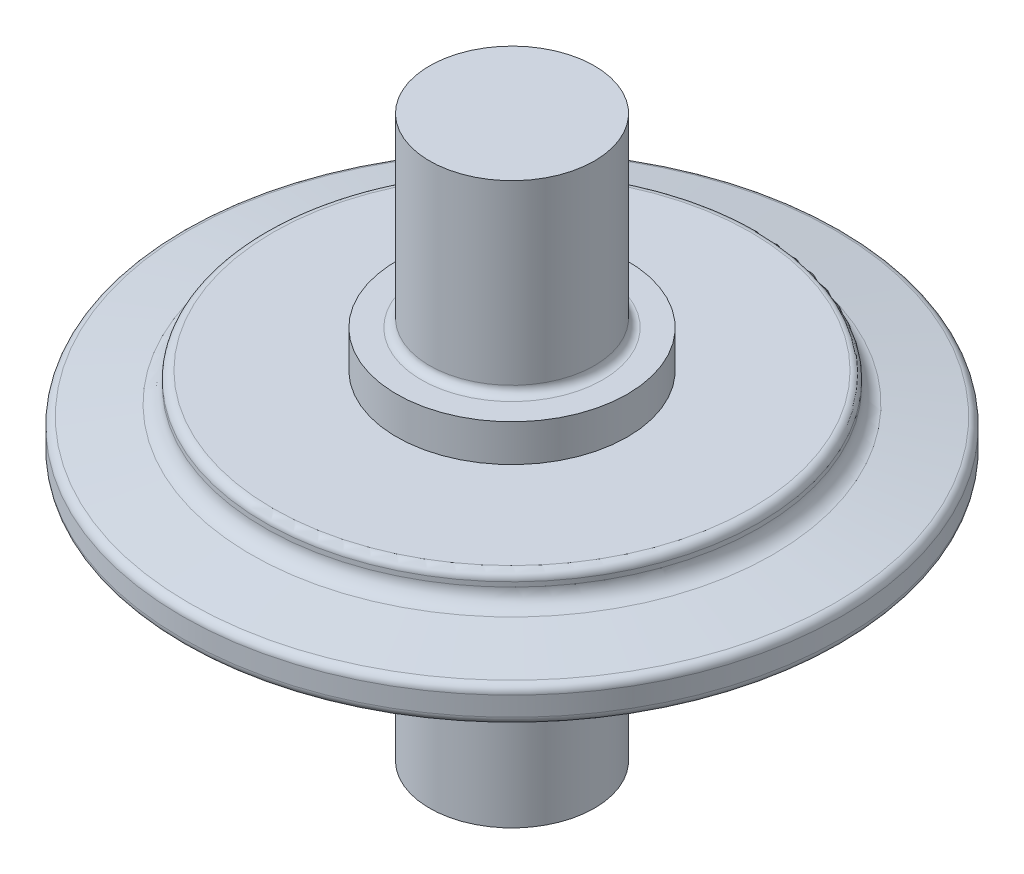
SolidWorks part; units mm, degrees
ref_plane "Front Plane" through (0, 0, 0) normal (0, 0, 1) x (1, 0, 0)
ref_plane "Top Plane" through (0, 0, 0) normal (0, 1, 0) x (1, 0, 0)
ref_plane "Right Plane" through (0, 0, 0) normal (1, 0, 0) x (0, 0, -1)
sketch "Sketch1" plane through (0, 0, 0) normal (0, 0, 1) x (1, 0, 0)
  line L0 (249.7318, 31.6679) -> (249.7318, 29.346)
  line L1 (258.0791, 33.9788) -> (250.5581, 32.6527)
  line L2 (250.5581, 28.3612) -> (258.0791, 27.0351)
  line L3 (259.7318, 25.0655) -> (259.7318, 24.507)
  line L4 (259.7318, 36.507) -> (259.7318, 35.9484)
  line L5 (275.7318, 23.507) -> (275.7318, 19.007)
  line L6 (275.7318, 42.007) -> (275.7318, 37.507)
  line L7 (279.7318, 18.007) -> (279.7318, -3.493)
  line L8 (279.7318, 64.507) -> (279.7318, 43.007)
  line L9 (289.7318, 64.507) -> (279.7318, 64.507)
  line L10 (289.7318, -3.493) -> (279.7318, -3.493)
  line L11 (289.7318, -3.493) -> (289.7318, 64.507)
  line L12 (260.7318, 23.507) -> (275.7318, 23.507)
  line L13 (260.7318, 37.507) -> (275.7318, 37.507)
  line L14 (275.7318, 19.007) -> (278.7318, 19.007)
  line L15 (275.7318, 42.007) -> (278.7318, 42.007)
  arc A1 (249.7318, 29.346) -> (250.5581, 28.3612) centre (250.7318, 29.346) ccw
  arc A2 (250.5581, 32.6527) -> (249.7318, 31.6679) centre (250.7318, 31.6679) ccw
  arc A3 (259.7318, 25.0655) -> (258.0791, 27.0351) centre (257.7318, 25.0655) ccw
  arc A4 (258.0791, 33.9788) -> (259.7318, 35.9484) centre (257.7318, 35.9484) ccw
  arc A5 (260.7318, 37.507) -> (259.7318, 36.507) centre (260.7318, 36.507) ccw
  arc A6 (259.7318, 24.507) -> (260.7318, 23.507) centre (260.7318, 24.507) ccw
  arc A7 (278.7318, 42.007) -> (279.7318, 43.007) centre (278.7318, 43.007) ccw
  arc A8 (279.7318, 18.007) -> (278.7318, 19.007) centre (278.7318, 18.007) ccw
revolve "Revolve1" add sketch "Sketch1" angle 360 about L11
